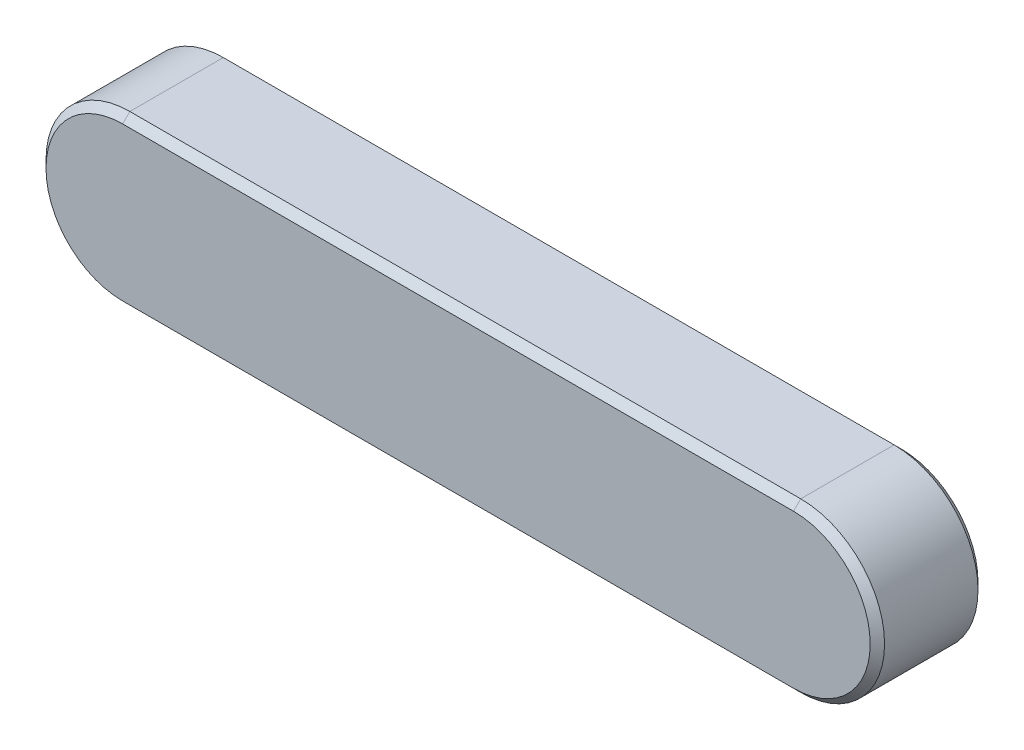
from build123d import *

# Parameters (mm, degrees)
BASEKEY_DEPTH = 4.5
CHAMFER1_SIZE = 0.6


with BuildPart() as part:
    # Sketch1 → BaseKey (new, symmetric)
    with BuildSketch(Plane.XY):
        with BuildLine():
            Line((-56, 7), (0, 7))
            ThreePointArc((0, 7), (7, 0), (0, -7))
            Line((0, -7), (-56, -7))
            ThreePointArc((-56, -7), (-63, 0), (-56, 7))
        make_face()
    extrude(amount=BASEKEY_DEPTH, both=True)

    # Chamfer1
    chamfer1_edges = [part.edges().sort_by_distance(p)[0] for p in [
        (7, 0, 4.5),
        (-28, 7, 4.5),
        (-63, 0, 4.5),
        (-28, 7, -4.5),
        (7, 0, -4.5),
        (-28, -7, -4.5),
        (-63, 0, -4.5),
        (-28, -7, 4.5),
    ]]
    chamfer(chamfer1_edges, length=CHAMFER1_SIZE)


solid = part.part
